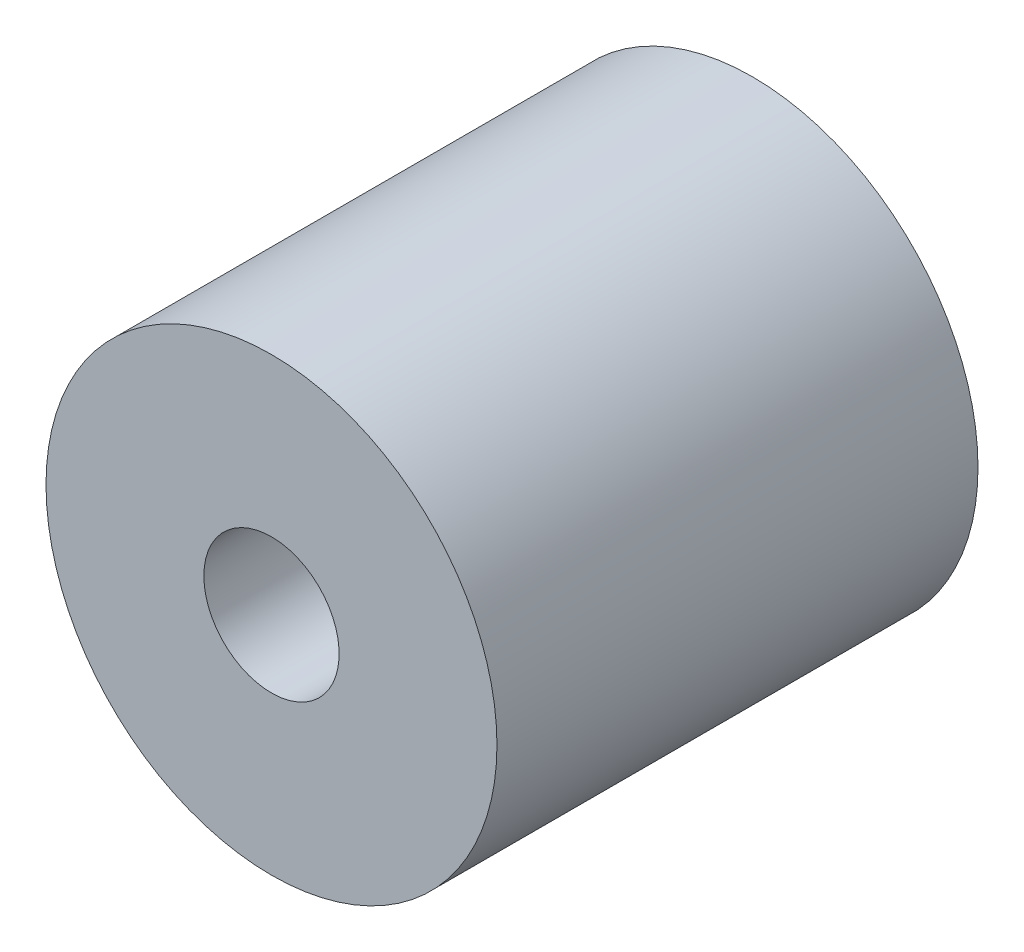
SolidWorks part; units mm, degrees
material "优力胶"
ref_plane "前视基准面" through (0, 0, 0) normal (0, 0, 1) x (1, 0, 0)
ref_plane "上视基准面" through (0, 0, 0) normal (0, 1, 0) x (1, 0, 0)
ref_plane "右视基准面" through (0, 0, 0) normal (1, 0, 0) x (0, 0, -1)
sketch "草图1" plane through (0, 0, 0) normal (0, 0, 1) x (1, 0, 0)
  circle A0 centre (0, 0) radius 7.5
  dimension "D1" = 15
extrude "凸台-拉伸1" add sketch "草图1" along normal blind 16
hole_wizard "M4 六角凹头螺钉的柱形沉头孔1" positions "草图3" profile "草图2" counterbore size "M4" standard "ISO" end condition through all
sketch "草图3" plane through (0, 0, 0) normal (0, 0, -1) x (-1, 0, 0)
  point P0 (0, 0)
sketch "草图2" plane through (0, 0, 0) normal (1, 0, 0) x (0, 1, 0)
  line L0 (0, 0) -> (0, 16)
  line L1 (0, 16) -> (2.25, 16)
  line L3 (2.25, 16) -> (2.25, 12)
  line L4 (2.25, 12) -> (4.5, 12)
  line L5 (4.5, 12) -> (4.5, 0)
  line L7 (4.5, 0) -> (0, 0)
  line L11 (0, -6.35) -> (0, 107.95) construction
  dimension "通孔孔直径" = 4.5
  dimension "通孔孔深度" = 16
  dimension "柱形沉头孔直径" = 9
  dimension "柱形沉头孔深度" = 12
chamfer "倒角1" distance 1 angle 45 1 edges at (-4.5, 0, 0)
